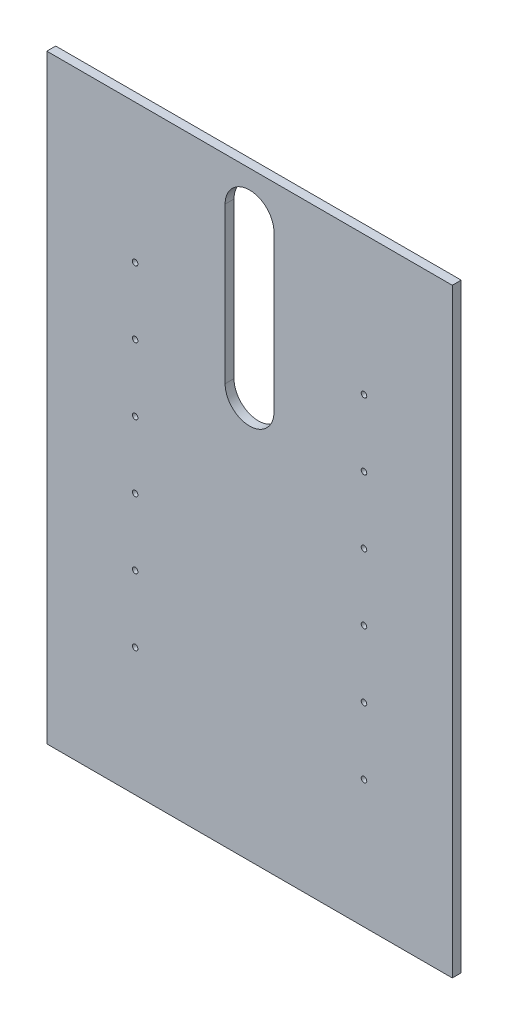
from build123d import *

# Parameters (mm, degrees)
SKETCH1_W           = 365
SKETCH1_H           = 540
BOSS_EXTRUDE1_DEPTH = 8
M6_TAPPED_HOLE1_D   = 5
LPATTERN1_COUNT     = 6
LPATTERN1_PITCH     = 60


with BuildPart() as part:
    # Sketch1 → Boss-Extrude1 (new body)
    with BuildSketch(Plane.XY):
        with Locations((182.5, -270)):
            Rectangle(SKETCH1_W, SKETCH1_H)
        with BuildLine():
            Line((204.5, -39), (204.5, -179))
            ThreePointArc((204.5, -179), (182.5, -201), (160.5, -179))
            Line((160.5, -179), (160.5, -39))
            ThreePointArc((160.5, -39), (182.5, -17), (204.5, -39))
        make_face(mode=Mode.SUBTRACT)
    extrude(amount=BOSS_EXTRUDE1_DEPTH)

    # M6 Tapped Hole1 (through all)
    with Locations(Plane.XY.offset(8)):
        with Locations((79.5, -125), (285.5, -125)):
            m6_tapped_hole1 = Hole(M6_TAPPED_HOLE1_D / 2)

    # LPattern1: M6 Tapped Hole1 ×6
    with Locations(*[(0, -i * LPATTERN1_PITCH, 0) for i in range(1, LPATTERN1_COUNT)]):
        add(m6_tapped_hole1, mode=Mode.SUBTRACT)


solid = part.part
